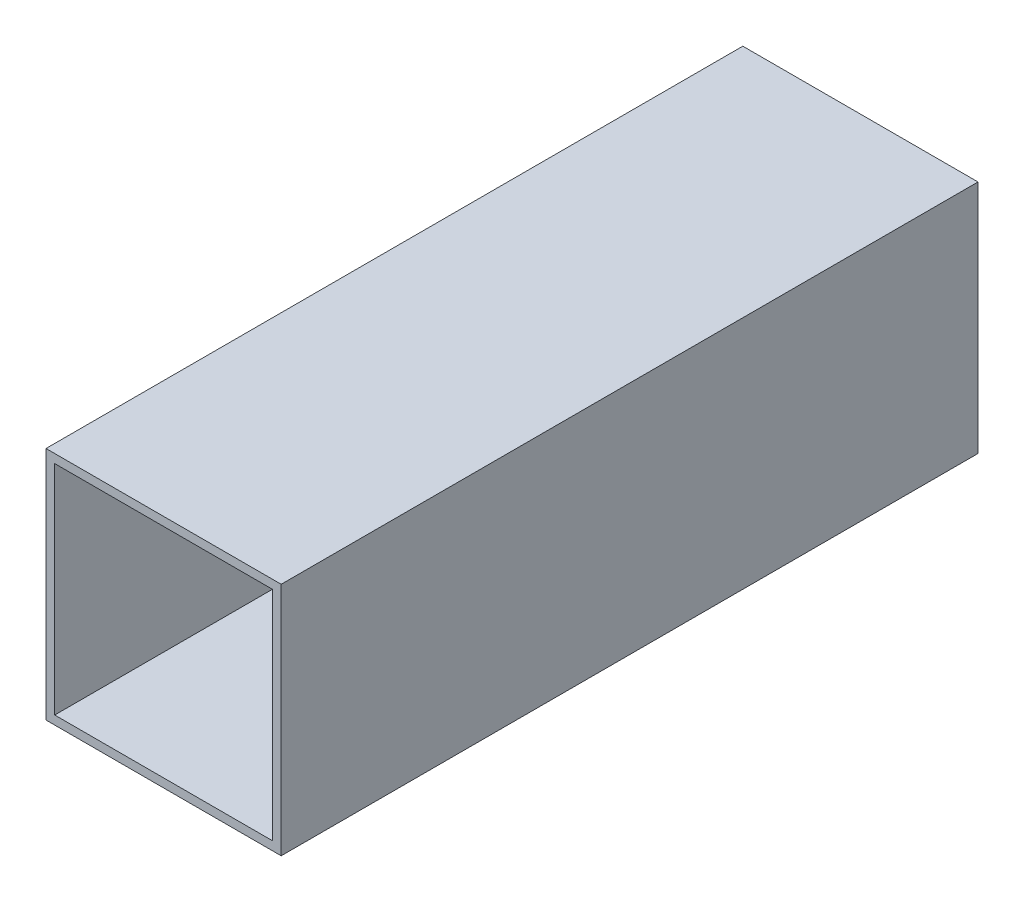
from build123d import *

# Parameters (mm, degrees)
SKETCH1_W           = 270
SKETCH1_H           = 270
SKETCH1_W_2         = 250
SKETCH1_H_2         = 250
EXTRUDE_THIN1_DEPTH = 800


with BuildPart() as part:
    # Sketch1 → Extrude-Thin1 (new body)
    with BuildSketch(Plane.XY):
        Rectangle(SKETCH1_W, SKETCH1_H)
        Rectangle(SKETCH1_W_2, SKETCH1_H_2, mode=Mode.SUBTRACT)
    extrude(amount=EXTRUDE_THIN1_DEPTH)


solid = part.part
